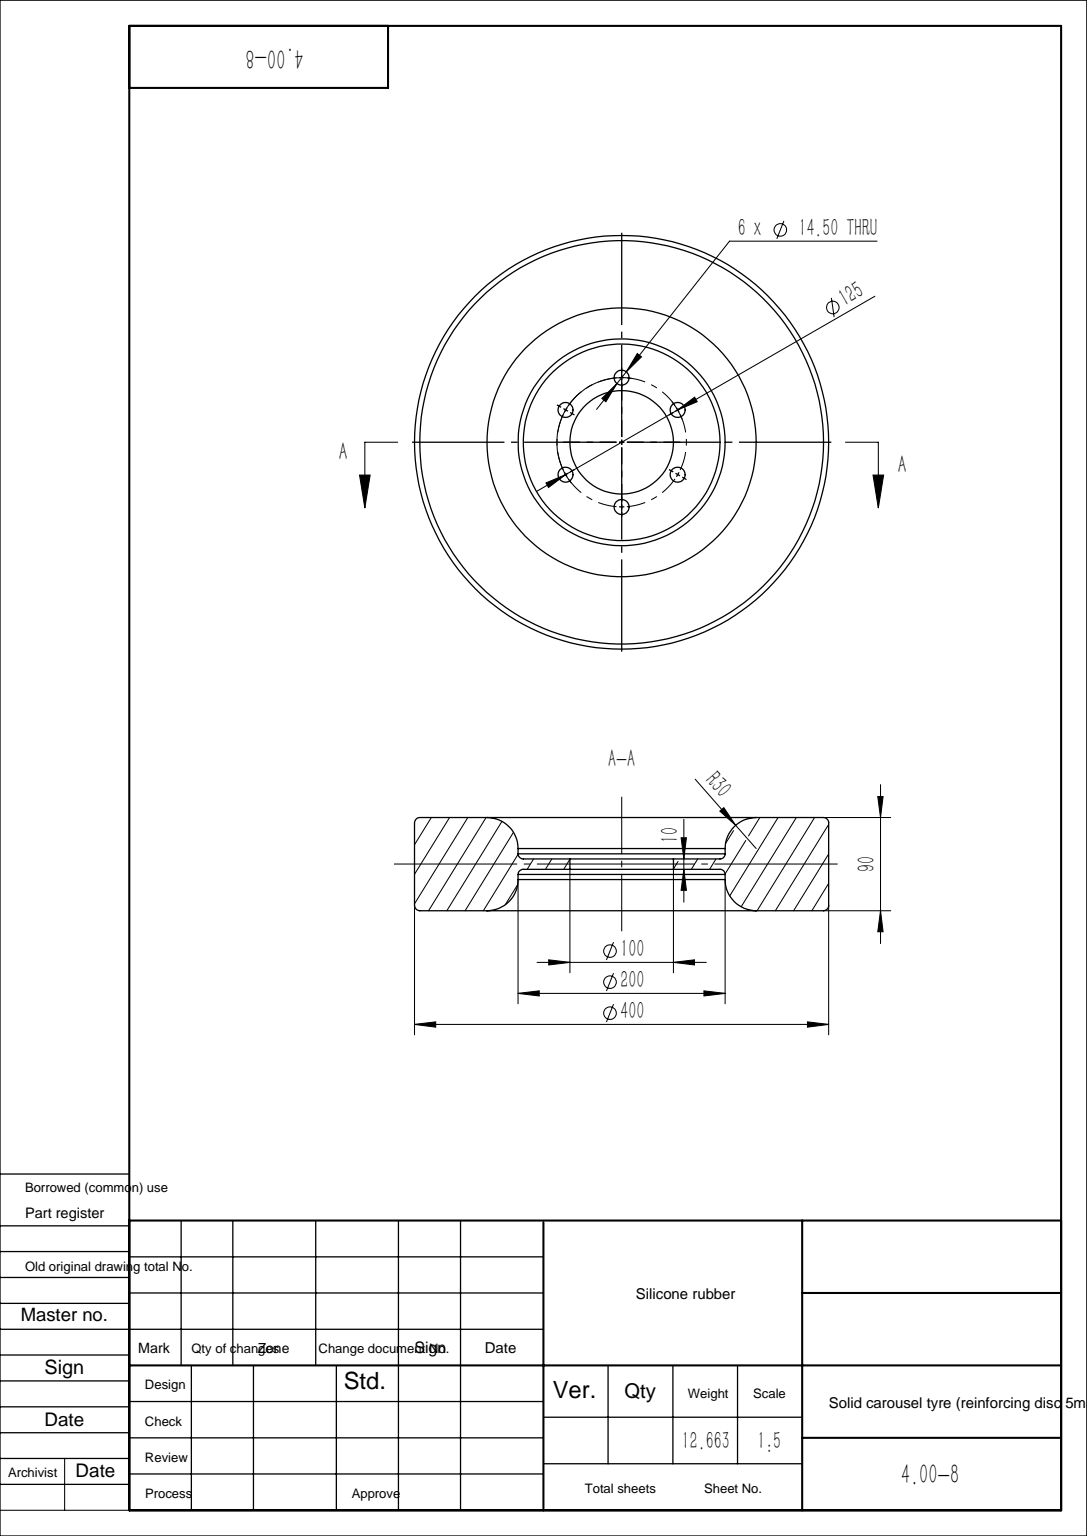
SolidWorks part; units mm, degrees
material "Silicone Rubber"
ref_plane "Front Plane" through (0, 0, 0) normal (0, 0, 1) x (1, 0, 0)
ref_plane "Top Plane" through (0, 0, 0) normal (0, 1, 0) x (1, 0, 0)
ref_plane "Right Plane" through (0, 0, 0) normal (1, 0, 0) x (0, 0, -1)
sketch "Sketch2" plane through (0, 0, 0) normal (0, 1, 0) x (1, 0, 0)
  line L0 (50, -5) -> (50, 5)
  line L1 (50, 5) -> (100, 5)
  line L2 (100, 5) -> (100, 15)
  line L3 (130, 45) -> (200, 45)
  line L4 (200, 45) -> (200, -45)
  line L5 (200, 0) -> (50, 0) construction
  line L6 (0, 0) -> (0, 50.7751) construction
  line L7 (130, -45) -> (200, -45)
  line L8 (100, -5) -> (100, -15)
  line L9 (50, -5) -> (100, -5)
  arc A0 (100, 15) -> (130, 45) centre (130, 15) cw
  arc A1 (100, -15) -> (130, -45) centre (130, -15) ccw
  dimension "D1" = 100
  dimension "D5" = 30
  dimension "D2" = 200
  dimension "D3" = 400
  dimension "D4" = 90
  dimension "D6" = 10
revolve "Revolve1" add sketch "Sketch2" angle 360 about L6
fillet "Fillet1" radius 5 4 edges at (200, 0, -45) (200, 0, 45) (100, 0, -5) (100, 0, 5)
hole_wizard "Ø14.5 (14.5) Diameter Hole1" positions "Sketch3" profile "Sketch4" hole size "Ø14.5" standard "GB" end condition up to next
sketch "Sketch3" plane through (0, 0, 5) normal (0, 0, 1) x (1, 0, 0)
  circle A0 centre (0, 0) radius 62.5 construction
  point P0 (0, 62.5)
  point P10 (54.1266, 31.25)
  point P11 (54.1266, -31.25)
  point P12 (0, -62.5)
  point P13 (-54.1266, -31.25)
  point P14 (-54.1266, 31.25)
  dimension "D1" = 125
  dimension "D2" = 6
sketch "Sketch4" plane through (0, 62.5, 5) normal (1, 0, 0) x (0, -1, 0)
  line L0 (0, 0) -> (0, 10)
  line L1 (0, 10) -> (7.25, 10)
  line L2 (7.25, 10) -> (7.25, 0)
  line L5 (7.25, 0) -> (0, 0)
  line L11 (0, -6.35) -> (0, 107.95) construction
  dimension "通孔孔直径" = 14.5
  dimension "通孔孔深度" = 10
